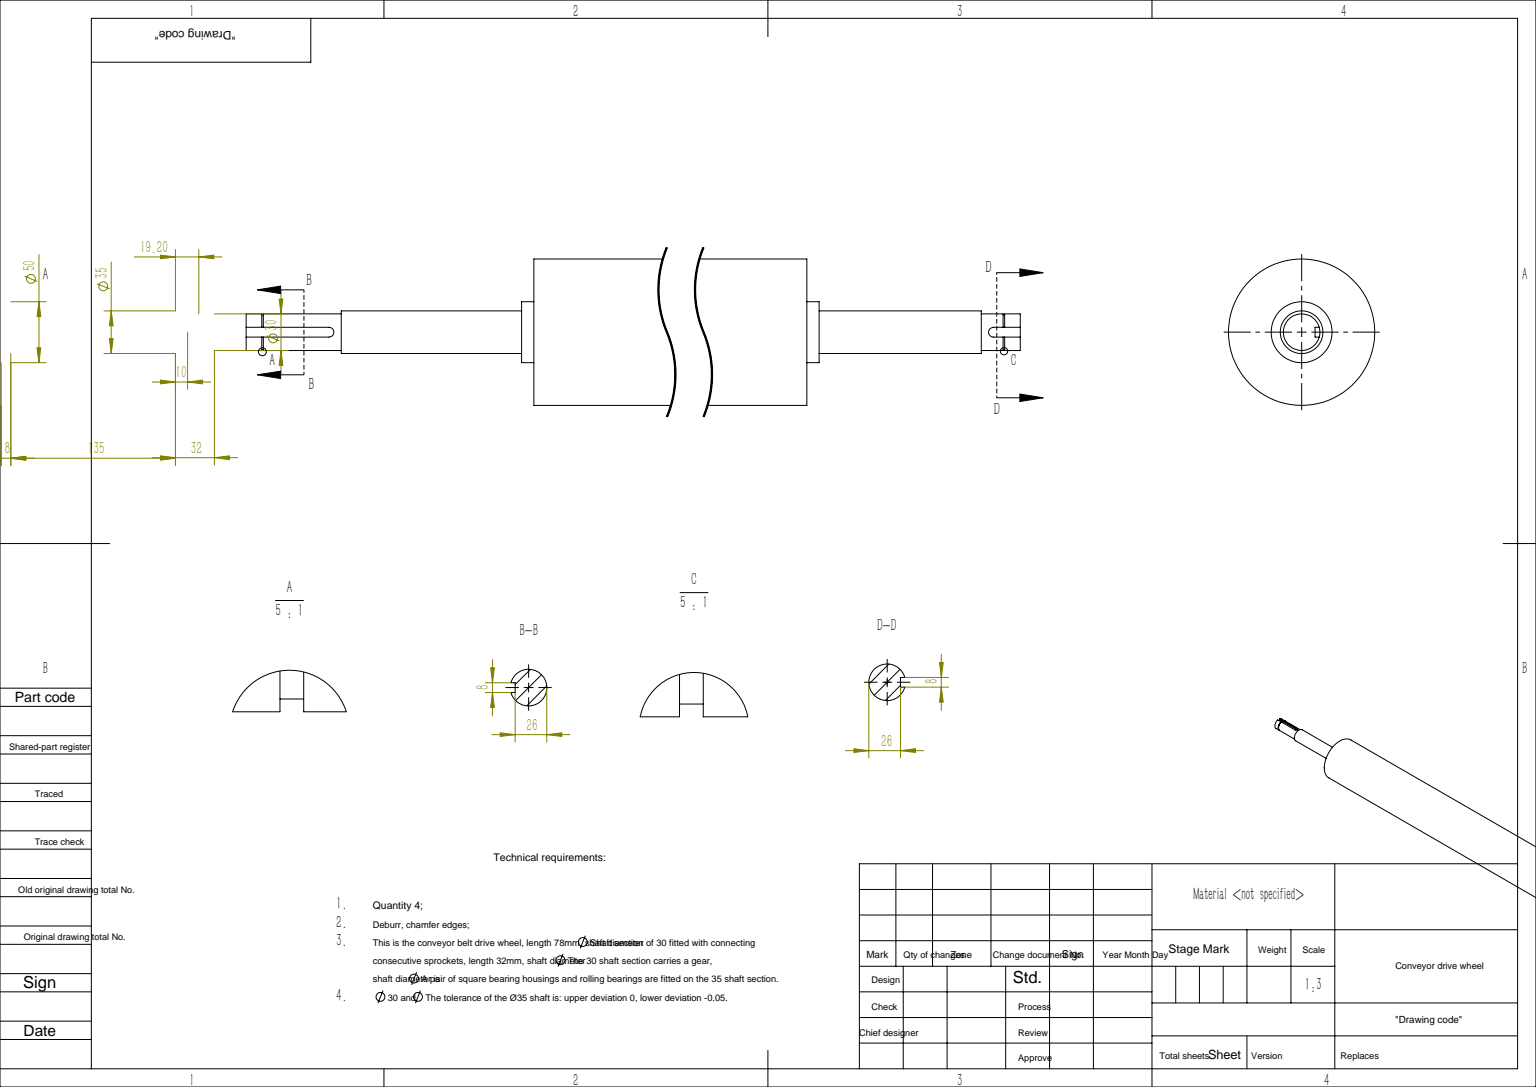
SolidWorks part; units mm, degrees
ref_plane "前视基准面" through (0, 0, 0) normal (0, 0, 1) x (1, 0, 0)
ref_plane "上视基准面" through (0, 0, 0) normal (0, 1, 0) x (1, 0, 0)
ref_plane "右视基准面" through (0, 0, 0) normal (1, 0, 0) x (0, 0, -1)
sketch "草图1" plane through (0, 0, 0) normal (0, 0, 1) x (1, 0, 0)
  line L0 (0, 0) -> (0, 15)
  line L1 (0, 15) -> (78, 15)
  line L2 (78, 15) -> (78, 17.5)
  line L3 (78, 17.5) -> (226, 17.5)
  line L4 (226, 17.5) -> (226, 25)
  line L5 (226, 25) -> (236, 25)
  line L6 (0, 0) -> (1261, 0)
  line L7 (236, 25) -> (236, 60)
  line L8 (236, 60) -> (1086, 60)
  line L9 (1086, 60) -> (1086, 25)
  line L10 (1086, 25) -> (1096, 25)
  line L11 (1096, 25) -> (1096, 17.5)
  line L12 (1096, 17.5) -> (1229, 17.5)
  line L13 (1229, 17.5) -> (1229, 15)
  line L14 (1229, 15) -> (1261, 15)
  line L15 (1261, 15) -> (1261, 0)
  dimension "D1" = 78
  dimension "D2" = 15
  dimension "D3" = 17.5
  dimension "D4" = 148
  dimension "D5" = 10
  dimension "D6" = 25
  dimension "D7" = 60
  dimension "D8" = 850
  dimension "D9" = 10
  dimension "D10" = 25
  dimension "D11" = 17.5
  dimension "D12" = 133
  dimension "D13" = 32
  dimension "D14" = 15
revolve "旋转1" add sketch "草图1" angle 360 about L6
ref_plane "基准面1" through (0, 15, 0) normal (0, 1, 0) x (1, 0, 0)
sketch "草图2" plane through (0, 15, 0) normal (0, 1, 0) x (1, 0, 0)
  line L0 (0, 0) -> (78, 0) construction
  line L1 (78, 17.5) -> (78, -17.5) construction
  line L2 (68, 4) -> (-10, 4)
  line L3 (-10, 4) -> (-10, -4)
  line L4 (-10, -4) -> (68, -4)
  line L5 (78, 15) -> (78, -15) construction
  line L6 (0, 15) -> (0, -15) construction
  arc A0 (68, -4) -> (68, 4) centre (68, 0) ccw
  dimension "D1" = 4
  dimension "D2" = 10
  dimension "D3" = 10
extrude "切除-拉伸1" cut sketch "草图2" against normal blind 4
ref_plane "基准面2" through (12.8, 0, 0) normal (-1, 0, 0) x (0, 0, 1)
sketch "草图3" plane through (12.8, 0, 0) normal (-1, 0, 0) x (0, 0, 1)
  circle A0 centre (0, 0) radius 15
  arc A2 (-4, 14.4568) -> (4, 14.4568) centre (0, 0) ccw construction
  circle A3 centre (0, 0) radius 14.3
  dimension "D1" = 28.6
extrude "切除-拉伸2" cut sketch "草图3" against normal blind 1.3
ref_plane "基准面3" through (0, 15, 0) normal (0, 1, 0) x (1, 0, 0)
sketch "草图4" plane through (0, 15, 0) normal (0, 1, 0) x (1, 0, 0)
  line L0 (1229, 0) -> (1261, 0) construction
  line L1 (1229, -15) -> (1229, 15) construction
  line L2 (1261, -15) -> (1261, 15) construction
  line L3 (1239, 4) -> (1271, 4)
  line L4 (1271, 4) -> (1271, -4)
  line L5 (1271, -4) -> (1239, -4)
  line L6 (1229, -17.5) -> (1229, 17.5) construction
  arc A0 (1239, 4) -> (1239, -4) centre (1239, 0) ccw
  dimension "D1" = 10
  dimension "D2" = 4
  dimension "D3" = 10
extrude "切除-拉伸3" cut sketch "草图4" against normal blind 4
ref_plane "基准面4" through (1248.2, 0, 0) normal (1, 0, 0) x (0, 0, -1)
sketch "草图5" plane through (1248.2, 0, 0) normal (1, 0, 0) x (0, 0, -1)
  circle A0 centre (0, 0) radius 15
  arc A1 (-4, 14.4568) -> (4, 14.4568) centre (0, 0) ccw construction
  circle A2 centre (0, 0) radius 14.3
  dimension "D1" = 28.6
extrude "切除-拉伸4" cut sketch "草图5" against normal blind 1.3
